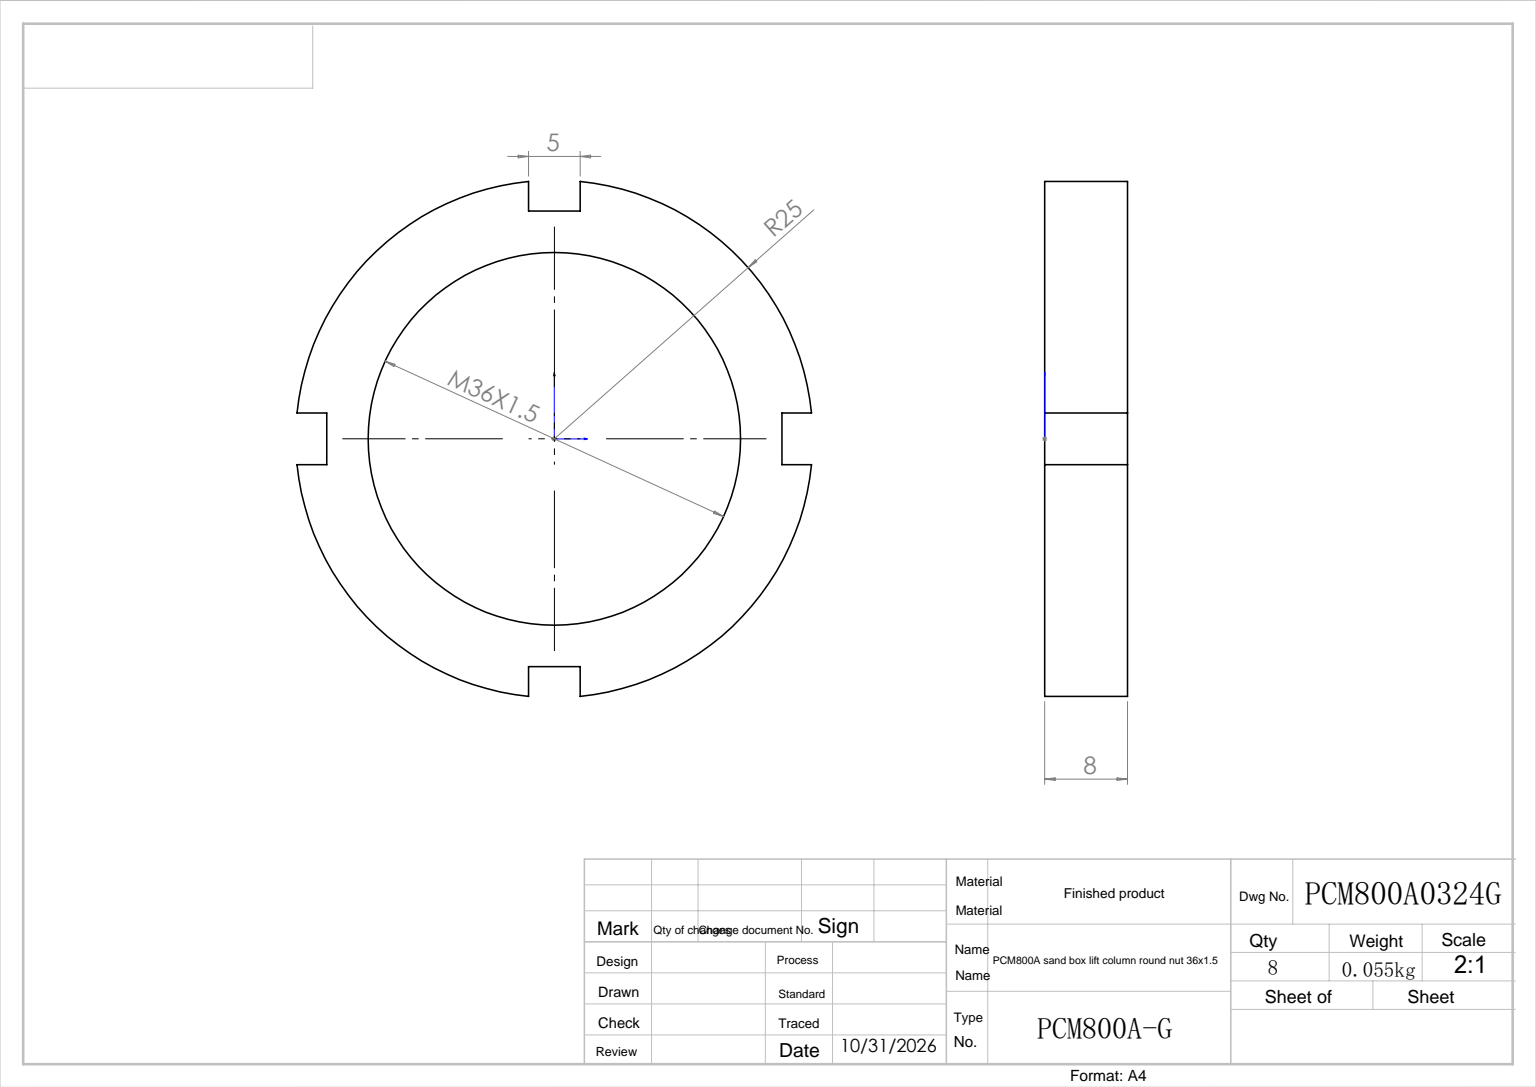
SolidWorks part; units mm, degrees
ref_plane "前视基准面" through (0, 0, 0) normal (0, 0, 1) x (1, 0, 0)
ref_plane "上视基准面" through (0, 0, 0) normal (0, 1, 0) x (1, 0, 0)
ref_plane "右视基准面" through (0, 0, 0) normal (1, 0, 0) x (0, 0, -1)
sketch "草图1" plane through (0, 0, 0) normal (0, 0, 1) x (1, 0, 0)
  line L0 (-2.5, 24.8711) -> (-2.5, 22)
  line L1 (-2.5, 22) -> (2.5, 22)
  line L2 (2.5, 22) -> (2.5, 24.8711)
  line L3 (0, 0) -> (28.0813, 0) construction
  line L4 (22, 2.5) -> (22, -2.5)
  line L5 (24.8711, 2.5) -> (22, 2.5)
  line L6 (22, -2.5) -> (24.8711, -2.5)
  line L7 (2.5, -22) -> (-2.5, -22)
  line L8 (2.5, -24.8711) -> (2.5, -22)
  line L9 (-2.5, -22) -> (-2.5, -24.8711)
  line L10 (-22, -2.5) -> (-22, 2.5)
  line L11 (-24.8711, -2.5) -> (-22, -2.5)
  line L12 (-22, 2.5) -> (-24.8711, 2.5)
  circle A0 centre (0, 0) radius 18
  arc A1 (-2.5, 24.8711) -> (-24.8711, 2.5) centre (0, 0) ccw
  arc A2 (-24.8711, -2.5) -> (-2.5, -24.8711) centre (0, 0) ccw
  arc A3 (2.5, -24.8711) -> (24.8711, -2.5) centre (0, 0) ccw
  arc A4 (24.8711, 2.5) -> (2.5, 24.8711) centre (0, 0) ccw
  dimension "D1" = 5
  dimension "D2" = 22
  dimension "D3" = 2.5
extrude "拉伸1" add sketch "草图1" along normal blind 8
